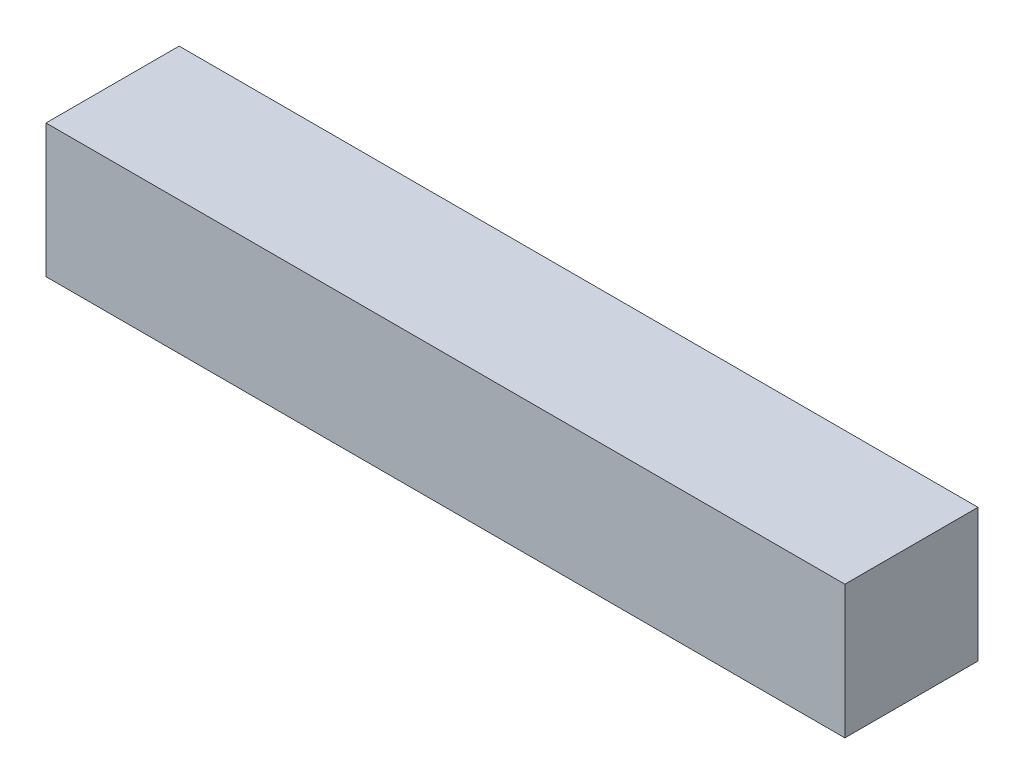
SolidWorks part; units mm, degrees
ref_plane "前视基准面" through (0, 0, 0) normal (0, 0, 1) x (1, 0, 0)
ref_plane "上视基准面" through (0, 0, 0) normal (0, 1, 0) x (1, 0, 0)
ref_plane "右视基准面" through (0, 0, 0) normal (1, 0, 0) x (0, 0, -1)
sketch "草图1" plane through (0, 0, 0) normal (1, 0, 0) x (0, 0, -1)
  line L1 (5, -5) -> (-5, -5)
  line L2 (5, -5) -> (5, 5)
  line L3 (5, 5) -> (-5, 5)
  line L4 (-5, -5) -> (-5, 5)
  line L5 (5, -5) -> (-5, 5) construction
  line L6 (5, 5) -> (-5, -5) construction
  point P0 (0, 0)
  dimension "D1" = 10
extrude "凸台-拉伸1" add sketch "草图1" along normal blind 60
